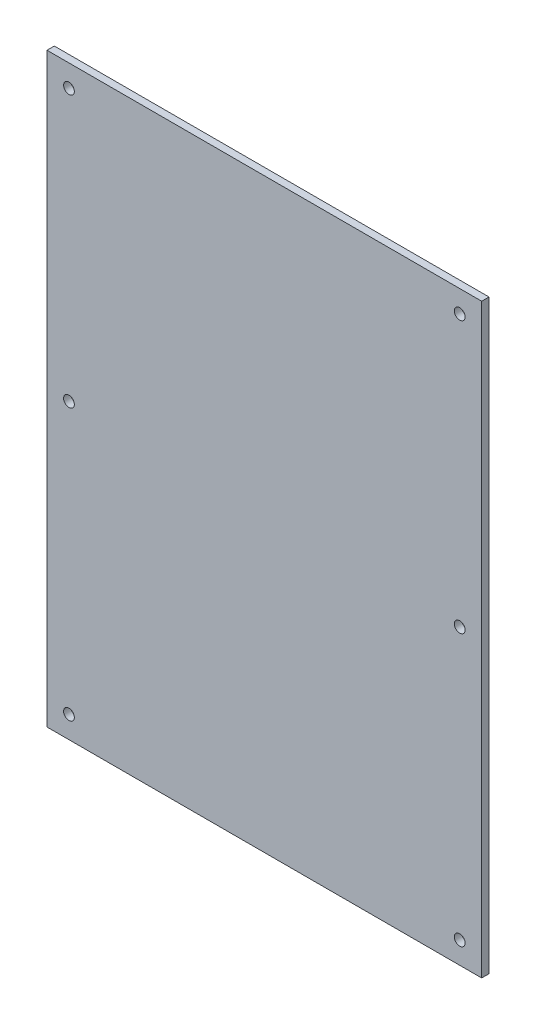
SolidWorks part; units mm, degrees
ref_plane "前视基准面" through (0, 0, 0) normal (0, 0, 1) x (1, 0, 0)
ref_plane "上视基准面" through (0, 0, 0) normal (0, 1, 0) x (1, 0, 0)
ref_plane "右视基准面" through (0, 0, 0) normal (1, 0, 0) x (0, 0, -1)
sketch "草图1" plane through (0, 0, 0) normal (0, 0, 1) x (1, 0, 0)
  line L1 (89, -120) -> (-89, -120)
  line L2 (89, -120) -> (89, 120)
  line L3 (89, 120) -> (-89, 120)
  line L4 (-89, -120) -> (-89, 120)
  line L5 (89, -120) -> (-89, 120) construction
  line L6 (89, 120) -> (-89, -120) construction
  point P0 (0, 0)
  dimension "D1" = 178
  dimension "D2" = 240
extrude "凸台-拉伸1" add sketch "草图1" along normal blind 3
sketch "草图2" plane through (0, 0, 3) normal (0, 0, 1) x (1, 0, 0)
  line L8 (-80, 111) -> (-80, -111)
  line L9 (-80, -111) -> (80, -111)
  line L10 (80, -111) -> (80, 111)
  line L11 (80, 111) -> (-80, 111)
  line L12 (-80, 111) -> (-80, -111) construction
  line L13 (-80, -111) -> (80, -111) construction
  line L14 (80, -111) -> (80, 111) construction
  line L15 (80, 111) -> (-80, 111) construction
  circle A0 centre (-80, 111) radius 2.2
  circle A1 centre (80, 111) radius 2.2
  circle A2 centre (80, -111) radius 2.2
  circle A3 centre (-80, -111) radius 2.2
  circle A4 centre (-80, 0) radius 2.2
  circle A5 centre (80, 0) radius 2.2
  dimension "D2" = 4.4
  dimension "D1" = 9
extrude "切除-拉伸1" cut sketch "草图2" against normal blind 10
